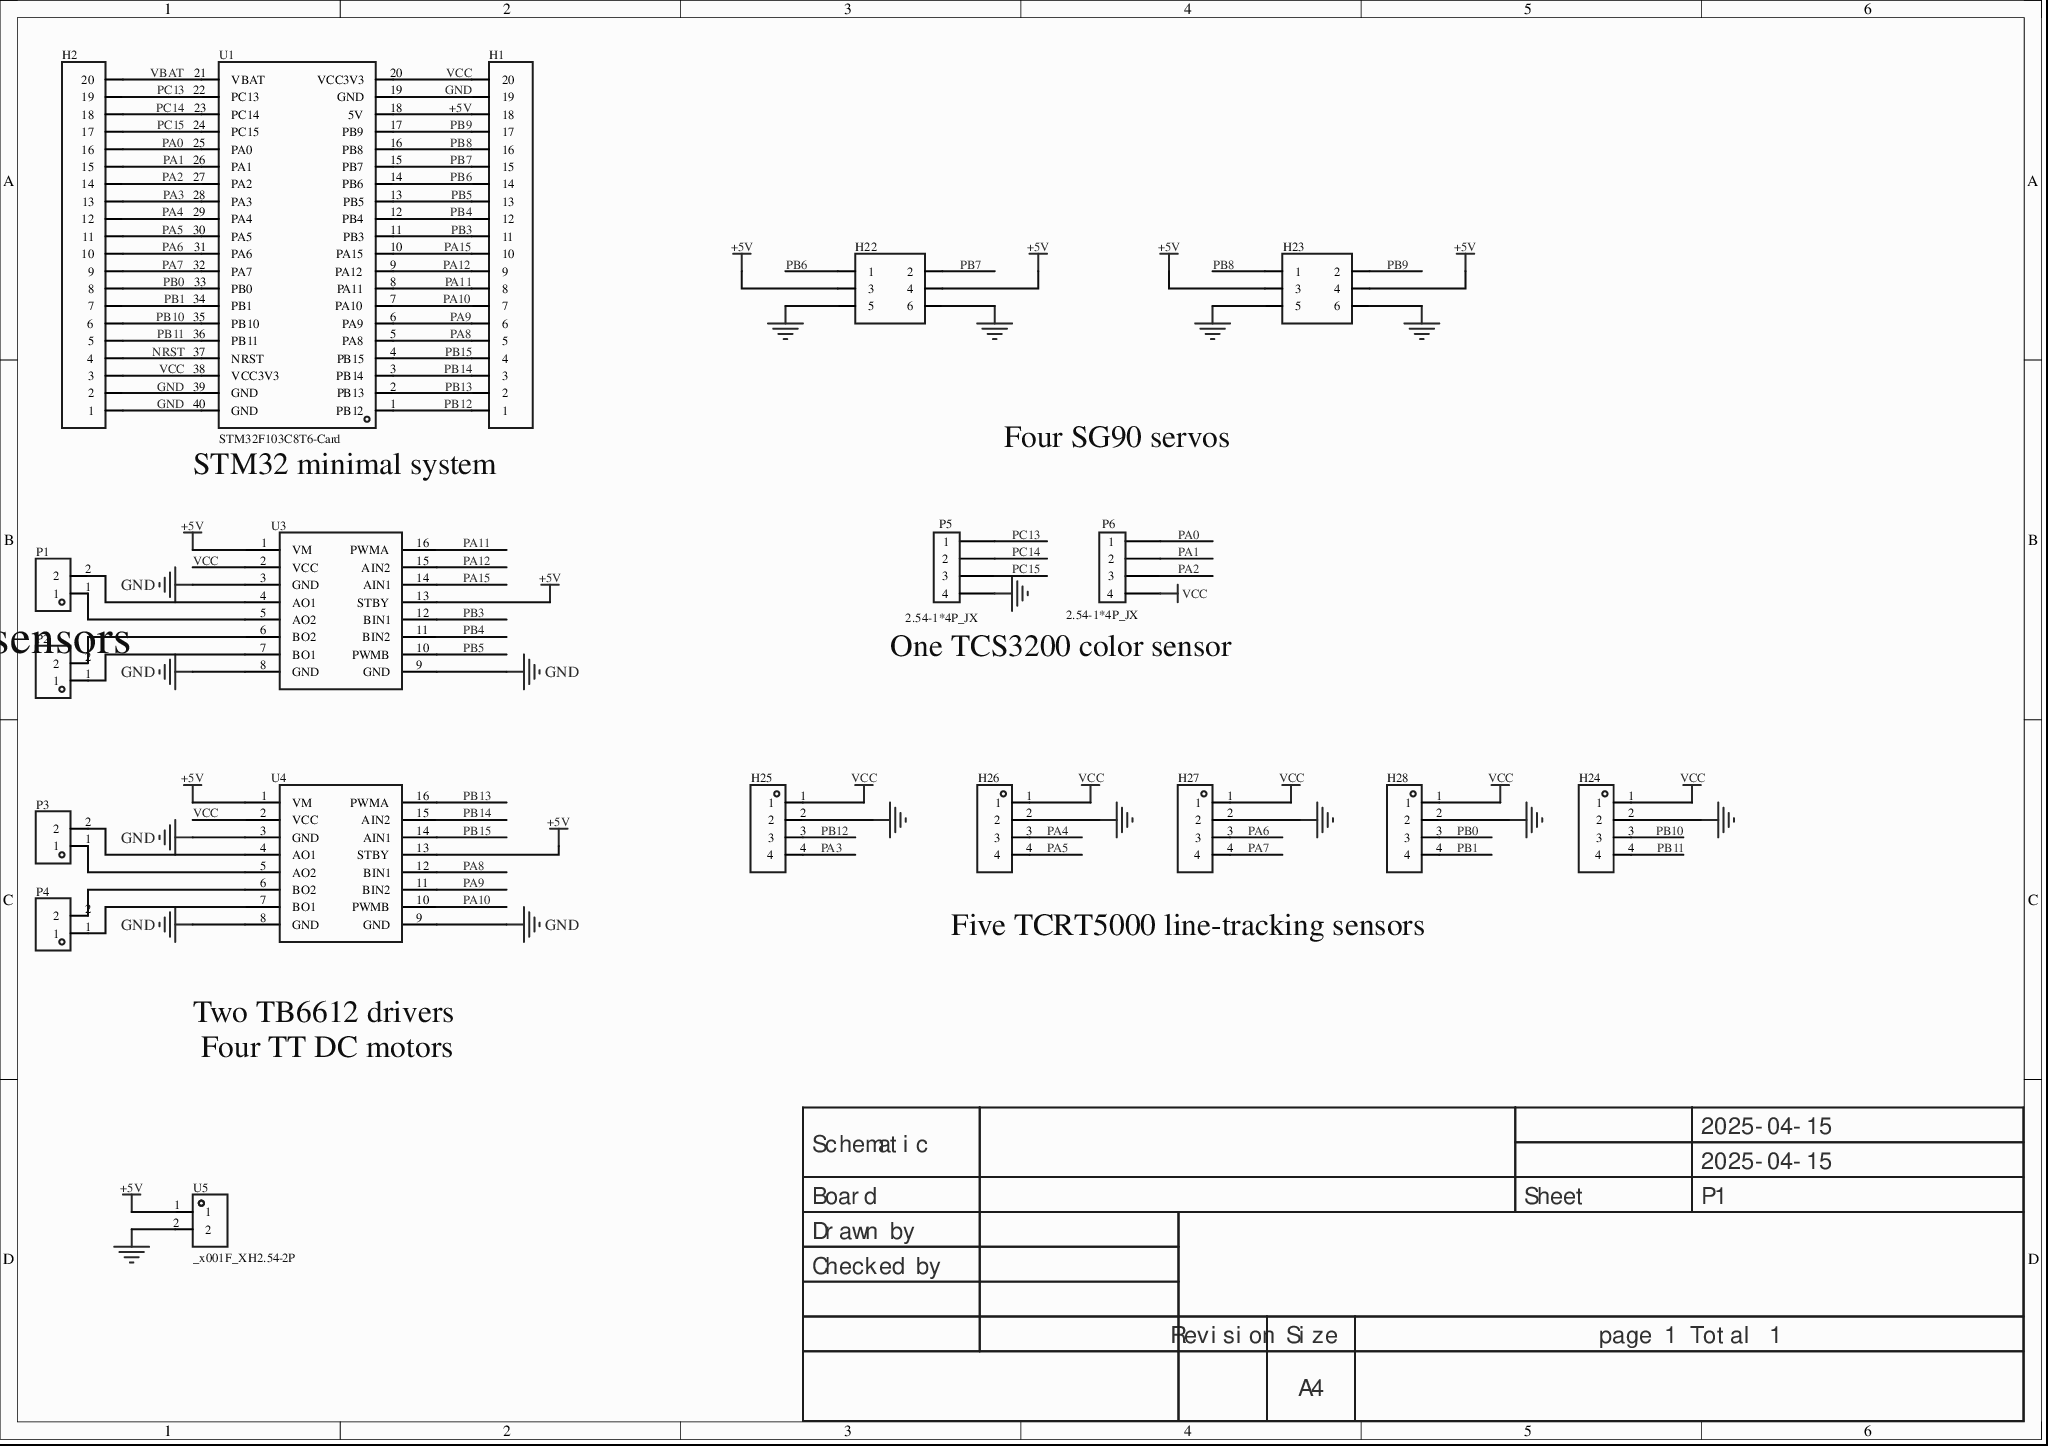
[diagram p0: MISC88999-3.schdoc]
# Altium project MISC88999-2.PrjPcb
1 sheet, 19 parts. Net scope: global (net labels, ports and power ports of the same name join across sheets).
Board file: MISC88999.pcbdoc

## Sheet MISC88999-3.schdoc
size 297 x 209 mm; Version: V1.0; @Project Name: MISC88999; @Page Count: 1; @Update Date: 2025-04-15; @Create Date: 2025-04-15; @Schematic Name: MISC88999; @Page No: 1; @Create Time: 16:30:37; @Update Time: 16:30:51; @Board Name: MISC88999

### Parts
H1  (no value)  [HDR-TH_20P-P2.54-V-F]
H2  (no value)  [HDR-TH_20P-P2.54-V-F]
H22  (no value)  [HDR-TH_6P-P2.54-V-F-R2-C3-S2.54]
H23  (no value)  [HDR-TH_6P-P2.54-V-F-R2-C3-S2.54]
H24  (no value)  [HDR-TH_4P-P2.54-V-M]
H25  (no value)  [HDR-TH_4P-P2.54-V-M]
H26  (no value)  [HDR-TH_4P-P2.54-V-M]
H27  (no value)  [HDR-TH_4P-P2.54-V-M]
H28  (no value)  [HDR-TH_4P-P2.54-V-M]
P1  KF301-2P terminal block  [CONN-TH_XY301V-A-5.0-2P]  (value not drawn)
P2  KF301-2P terminal block  [CONN-TH_XY301V-A-5.0-2P]  (value not drawn)
P3  KF301-2P terminal block  [CONN-TH_XY301V-A-5.0-2P]  (value not drawn)
P4  KF301-2P terminal block  [CONN-TH_XY301V-A-5.0-2P]  (value not drawn)
P5  2.54-1*4P_JX  [2.54-1*4P_JX]
P6  2.54-1*4P_JX  [2.54-1*4P_JX]
U1  STM32F103C8T6-Card  [CONN-TH_L53.3-W22.9_STM32F103C8T6-CARD]
U3  (no value)  [tb6612]
U4  (no value)  [tb6612]
U5  _x001F_XH2.54-2P  [CONN-TH_2P-P2.54-V]

### Nets
+5V: H1.18 H22.3 H22.4 H23.3 H23.4 U1.18(5V) U3.1(VM) U3.13(STBY) U4.1(VM) U4.13(STBY) U5.1
GND: H1.19 H2.1 H2.2 H22.5 H22.6 H23.5 H23.6 H24.2 H25.2 H26.2 H27.2 H28.2 P5.4 U1.19(GND) U1.39(GND) U1.40(GND) U3.3(GND) U3.8(GND) U3.9(GND) U4.3(GND) U4.8(GND) U4.9(GND) U5.2
VCC: H1.20 H2.3 H24.1 H25.1 H26.1 H27.1 H28.1 P6.4 U1.20(VCC3V3) U1.38(VCC3V3) U3.2(VCC) U4.2(VCC)
NRST: H2.4 U1.37(NRST)
PA0: H2.16 P6.1 U1.25(PA0)
PA1: H2.15 P6.2 U1.26(PA1)
PA2: H2.14 P6.3 U1.27(PA2)
PA3: H2.13 H25.4 U1.28(PA3)
PA4: H2.12 H26.3 U1.29(PA4)
PA5: H2.11 H26.4 U1.30(PA5)
PA6: H2.10 H27.3 U1.31(PA6)
PA7: H2.9 H27.4 U1.32(PA7)
PA8: H1.5 U1.5(PA8) U4.12(BIN1)
PA9: H1.6 U1.6(PA9) U4.11(BIN2)
PA10: H1.7 U1.7(PA10) U4.10(PWMB)
PA11: H1.8 U1.8(PA11) U3.16(PWMA)
PA12: H1.9 U1.9(PA12) U3.15(AIN2)
PA15: H1.10 U1.10(PA15) U3.14(AIN1)
PB0: H2.8 H28.3 U1.33(PB0)
PB1: H2.7 H28.4 U1.34(PB1)
PB3: H1.11 U1.11(PB3) U3.12(BIN1)
PB4: H1.12 U1.12(PB4) U3.11(BIN2)
PB5: H1.13 U1.13(PB5) U3.10(PWMB)
PB6: H1.14 H22.1 U1.14(PB6)
PB7: H1.15 H22.2 U1.15(PB7)
PB8: H1.16 H23.1 U1.16(PB8)
PB9: H1.17 H23.2 U1.17(PB9)
PB10: H2.6 H24.3 U1.35(PB10)
PB11: H2.5 H24.4 U1.36(PB11)
PB12: H1.1 H25.3 U1.1(PB12)
PB13: H1.2 U1.2(PB13) U4.16(PWMA)
PB14: H1.3 U1.3(PB14) U4.15(AIN2)
PB15: H1.4 U1.4(PB15) U4.14(AIN1)
PC13: H2.19 P5.1 U1.22(PC13)
PC14: H2.18 P5.2 U1.23(PC14)
PC15: H2.17 P5.3 U1.24(PC15)
VBAT: H2.20 U1.21(VBAT)
NetP1_1: P1.1 U3.5(AO2)
NetP1_2: P1.2 U3.4(AO1)
NetP2_1: P2.1 U3.7(BO1)
NetP2_2: P2.2 U3.6(BO2)
NetP3_1: P3.1 U4.5(AO2)
NetP3_2: P3.2 U4.4(AO1)
NetP4_1: P4.1 U4.7(BO1)
NetP4_2: P4.2 U4.6(BO2)

### Notes on the sheet
- Two TB6612 drivers,
  Four TT DC motors,
  Four SG90 servos,
  One TCS3200 color sensor,
  Two TCRT5000 line-tracking sensors
- STM32 minimal system
- Four SG90 servos
- One TCS3200 color sensor
- Five TCRT5000 line-tracking sensors
- (near U5) Two TB6612 drivers
  Four TT DC motors
- 2025-04-15
- Schematic
- Board
- Sheet
- P1
- Drawn by
- Checked by
- Revision
- Size
- A4
- page 1 Total 1

### Library data of the parts
H1 H2 = HDR-F_2.54_1x20P: ConvertToPcb: yes; ModelId: db7015f7ad9d48b8a3b1188db02e3429; ModelName: HDR-F-2.54_1x20; ModelTransform: 1999.996,100,0,0,0,0,0,0,-118.11; Device: HDR-F_2.54_1x20P; Symbol: HDR-F_2.54_1x20P; AddInBom: yes; SupplierPart: C50984; Supplier Footprint: 插件; FootprintName: HDR-TH_20P-P2.54-V-F
H22 H23 = HDR-F_2.54_2x3: Symbol: HDR-F-2.54_2x3; ConvertToPcb: yes; ModelId: 6dbaf143e10146ae9674d03402f6f9fb; ModelName: HDR-TH_6P-P2.54-F-LI-2X3P; ModelTransform: 315.7474,196.85,0,0,0,0,0,0,-125.984; Device: HDR-F_2.54_2x3; AddInBom: yes; SupplierPart: C92272; Supplier Footprint: 插件; FootprintName: HDR-TH_6P-P2.54-V-F-R2-C3-S2.54
H24-H28 = HDR-M_2.54_1x4P: Symbol: PZ254V-11-04P; ConvertToPcb: yes; ModelId: 112f4d05e8d64e99ab9a333894bea4f9; ModelName: HDR-TH_4P-P2.54-M-LI-1X4P; ModelTransform: 399.999,104.7242,0,0,0,0,0,0,-118.11; Device: HDR-M_2.54_1x4P; AddInBom: yes; SupplierPart: C492403; Supplier Footprint: 插件; FootprintName: HDR-TH_4P-P2.54-V-M
P1-P4 = KF301-2P接线端子: AddInBom: yes; ModelId: ef7ead88b0f2448d904975b26718870f; ModelTransform: 417.322,299.212,0,0,0,0,11.811,-7.835,-157.48; Symbol: KF301-2P terminal block; Device: KF301-2P terminal block; LCSC Part Name: KF301-2P接线端子; SupplierPart: C9900016950; ManufacturerPart: KF301-2P接线端子; Supplier Footprint: CK301-2P; Supplier: LCSC; ConvertToPcb: yes; FootprintName: CONN-TH_XY301V-A-5.0-2P; ModelName: CONN-TH_XY301V-A-5.0-2P
P5 P6 = C2337: Contributor: jixin002; Convert to PCB: yes; Origin Footprint: 2.54-1*4P_JX; Device: C2337; Symbol: 2.54-1*4P_JX; spicePre: P; Add into BOM: yes; ManufacturerPart: C2337; Supplier: EasyEDA; SupplierPart: C2337; FootprintName: 2.54-1*4P_JX
U1 = STM32F103C8T6-Card: AddInBom: yes; Symbol: STM32F103C8T6-CARD; Device: STM32F103C8T6-Card; LCSC Part Name: STM32F103C8T6-Card; SupplierPart: C9900077949; ManufacturerPart: STM32F103C8T6-Card; Supplier Footprint: 插件; Supplier: LCSC; ConvertToPcb: yes; FootprintName: CONN-TH_L53.3-W22.9_STM32F103C8T6-CARD
U3 U4 = tb6612: AddInBom: yes; Device: tb6612; ConvertToPcb: yes; JLCPCB Part Class: Extended library; SymbolName: tb6612; FootprintName: tb6612
U5 = _x001F_XH2.54-2P: AddInBom: yes; ModelId: 4b619f877c224111ac90f050b36c3583; ModelTransform: 295.275,224.409,0,180,0,0,0,17.717,-118.11; Symbol: _X001F_XH2.54-2P; Device: _x001F_XH2.54-2P; LCSC Part Name: _x001F_XH2.54-2P; SupplierPart: C9900016027; ManufacturerPart: _x001F_XH2.54-2P; Supplier Footprint: XH2.54-2P直插; JLCPCB Part Class: Extended library; Supplier: LCSC; ConvertToPcb: yes; FootprintName: CONN-TH_2P-P2.54-V; ModelName: CONN-TH_2P-P2.54-V